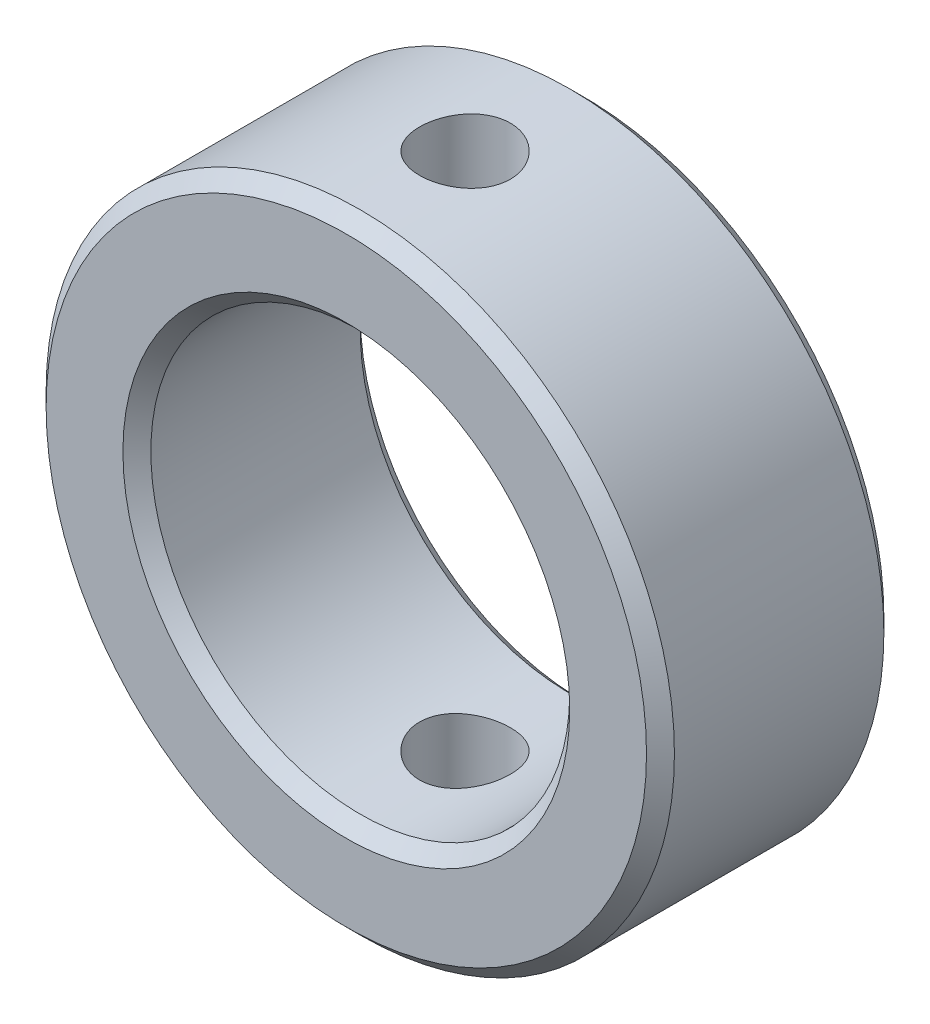
from build123d import *

# Parameters (mm, degrees)
SKETCH1_R               = 45
SKETCH1_R_2             = 30
BOSS_EXTRUDE1_DEPTH     = 34
CUT_EXTRUDE1_DEPTH      = 73.15261603
CUT_EXTRUDE1_DEPTH_BACK = 73.15261603
SKETCH2_R               = 6.5
CHAMFER1_SIZE           = 2


with BuildPart() as part:
    # Sketch1 → Boss-Extrude1 (new body)
    with BuildSketch(Plane.XY):
        Circle(SKETCH1_R)
        Circle(SKETCH1_R_2, mode=Mode.SUBTRACT)
    extrude(amount=BOSS_EXTRUDE1_DEPTH)

    # Sketch2 → Cut-Extrude1 (cut, two sides: drawn at the far end of the back side and taken through both)
    with BuildSketch(Plane(origin=(0, 0, 0), x_dir=(1, 0, 0), z_dir=(0, 1, 0)).offset(-CUT_EXTRUDE1_DEPTH_BACK)):
        with Locations(Location((0, -17, 0), (0, 0, 270))):
            Circle(SKETCH2_R)
    extrude(amount=CUT_EXTRUDE1_DEPTH + CUT_EXTRUDE1_DEPTH_BACK, mode=Mode.SUBTRACT)

    # Chamfer1
    chamfer1_edges = [part.edges().sort_by_distance(p)[0] for p in [
        (-45, 0, 0),
        (-45, 0, 34),
        (-30, 0, 0),
        (-30, 0, 34),
    ]]
    chamfer(chamfer1_edges, length=CHAMFER1_SIZE)


solid = part.part
